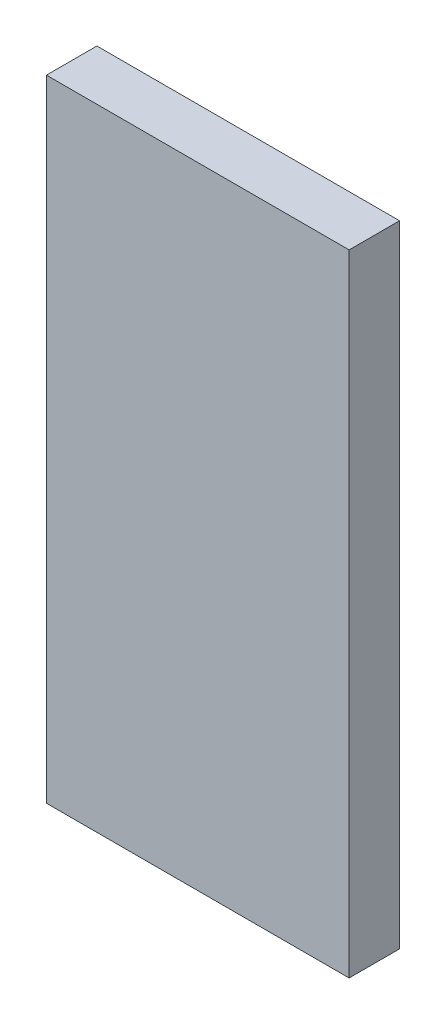
from build123d import *

# Parameters (mm, degrees)
SKETCH1_W      = 96
SKETCH1_H      = 200
EXTRUDE1_DEPTH = 8


with BuildPart() as part:
    # Sketch1 → Extrude1 (new, symmetric)
    with BuildSketch(Plane.XY):
        Rectangle(SKETCH1_W, SKETCH1_H)
    extrude(amount=EXTRUDE1_DEPTH, both=True)


solid = part.part
